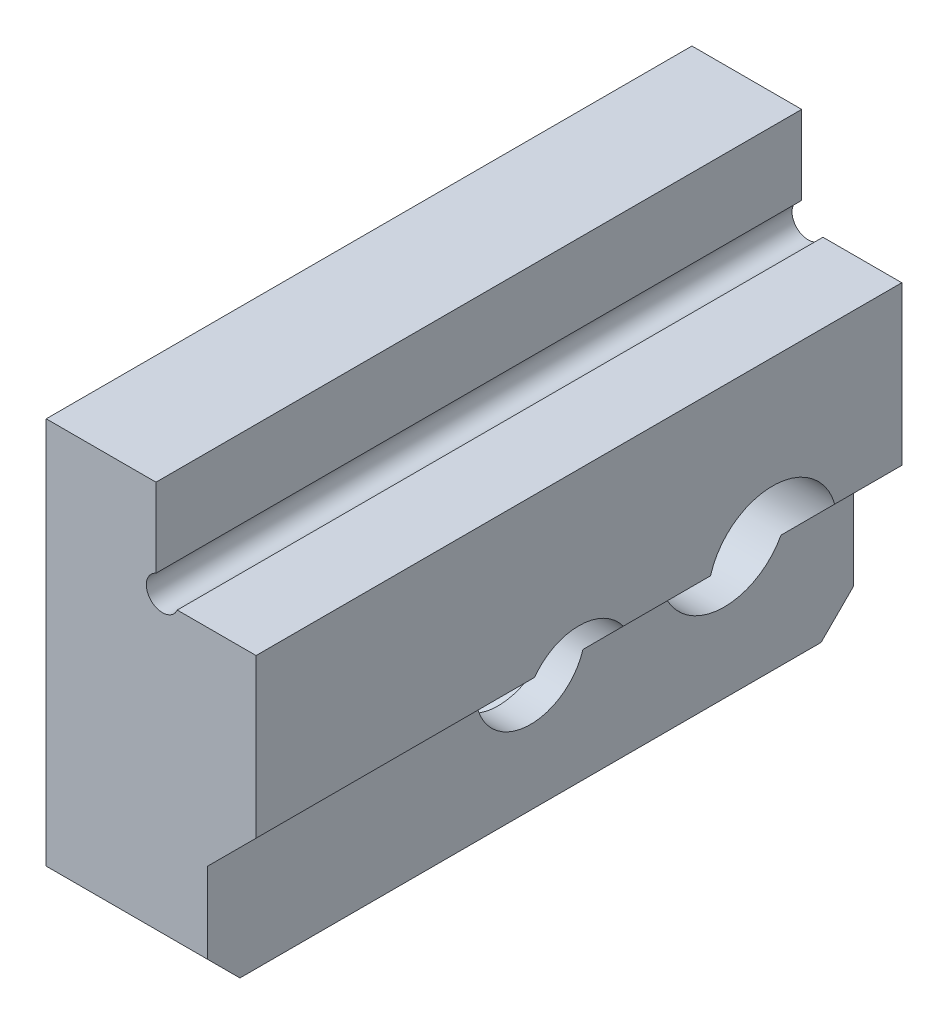
from build123d import *

# Parameters (mm, degrees)
BOSS_EXTRUDE1_DEPTH                                  = 20
CUT_EXTRUDE1_DEPTH                                   = 20
HOLE_SIZE_PER_SOCKET_HEAD_CAP_SCREW_TYPE_D           = 3.4
HOLE_SIZE_PER_SOCKET_HEAD_CAP_SCREW_TYPE_DEPTH       = 10
HOLE_SIZE_PER_SOCKET_HEAD_CAP_SCREW_TYPE_CBORE_D     = 6
HOLE_SIZE_PER_SOCKET_HEAD_CAP_SCREW_TYPE_CBORE_DEPTH = 4
HOLE_SIZE_PER_SOCKET_HEAD_CAP_SCREW_TYPE_TIP         = 1.021463052
CHAMFER1_SIZE                                        = 1
SKETCH8_R                                            = 2
CUT_EXTRUDE2_DEPTH                                   = 8


with BuildPart() as part:
    # Sketch1 → Boss-Extrude1 (new body)
    with BuildSketch(Plane.XY):
        with BuildLine():
            Line((0, 0), (0, 13))
            Line((0, 13), (3.4, 13))
            Line((3.4, 13), (3.4, 10.558257569))
            ThreePointArc((3.4, 10.558257569), (3.246446609, 9.746446609), (4.058257569, 9.9))
            Line((4.058257569, 9.9), (6.5, 9.9))
            Line((6.5, 9.9), (6.5, 0))
            Line((6.5, 0), (0, 0))
        make_face()
    extrude(amount=BOSS_EXTRUDE1_DEPTH)

    # Sketch7 → Cut-Extrude1 (cut)
    with BuildSketch(Plane.XY.offset(20)):
        Polygon((6.5, 5), (5, 3.5), (5, 0), (6.5, 0), align=None)
    extrude(amount=-CUT_EXTRUDE1_DEPTH, mode=Mode.SUBTRACT)

    # Hole size per socket head cap screw type 0
    with Locations(Plane(origin=(0, 0, 0), x_dir=(0, 0, -1), z_dir=(-1, 0, 0))):
        with Locations((-10, -4)):
            CounterBoreHole(HOLE_SIZE_PER_SOCKET_HEAD_CAP_SCREW_TYPE_D / 2, HOLE_SIZE_PER_SOCKET_HEAD_CAP_SCREW_TYPE_CBORE_D / 2, HOLE_SIZE_PER_SOCKET_HEAD_CAP_SCREW_TYPE_CBORE_DEPTH, depth=HOLE_SIZE_PER_SOCKET_HEAD_CAP_SCREW_TYPE_DEPTH)
            with Locations((0, 0, -(HOLE_SIZE_PER_SOCKET_HEAD_CAP_SCREW_TYPE_DEPTH + HOLE_SIZE_PER_SOCKET_HEAD_CAP_SCREW_TYPE_TIP / 2))):  # 118° drill point
                Cone(0, HOLE_SIZE_PER_SOCKET_HEAD_CAP_SCREW_TYPE_D / 2, HOLE_SIZE_PER_SOCKET_HEAD_CAP_SCREW_TYPE_TIP, mode=Mode.SUBTRACT)

    # Chamfer1
    chamfer1_edges = [part.edges().sort_by_distance(p)[0] for p in [
        (2.5, 0, 20),
        (2.5, 0, 0),
    ]]
    chamfer(chamfer1_edges, length=CHAMFER1_SIZE)

    # Sketch8 → Cut-Extrude2 (cut)
    with BuildSketch(Plane.ZY):
        with Locations((4, 4.45)):
            Circle(SKETCH8_R)
    extrude(amount=-CUT_EXTRUDE2_DEPTH, mode=Mode.SUBTRACT)


solid = part.part
